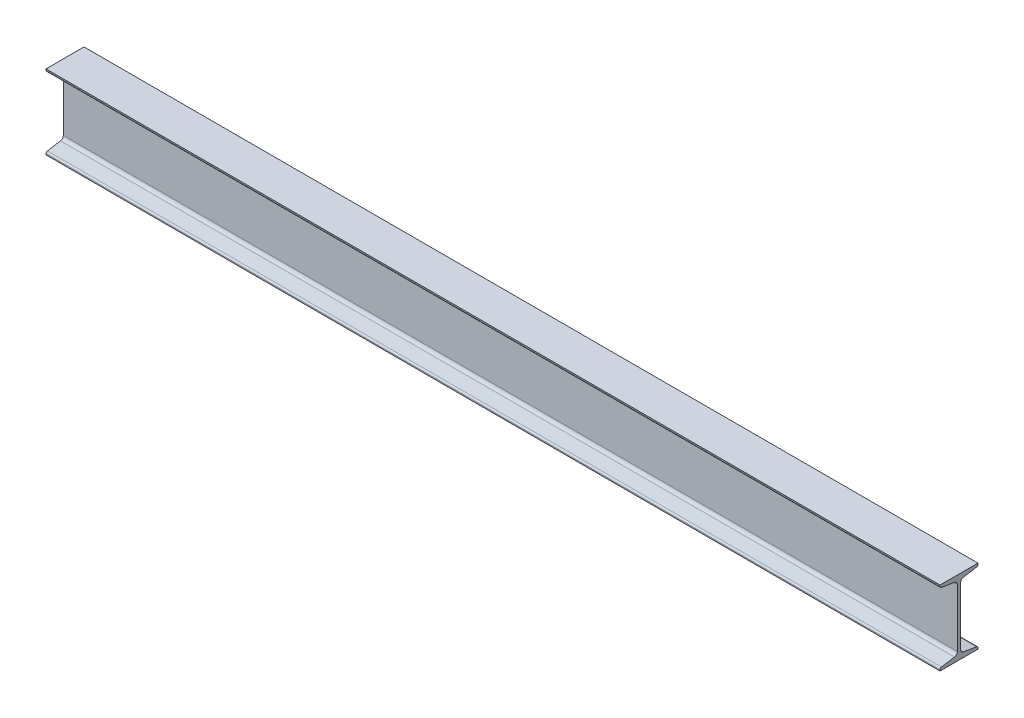
from build123d import *

# Parameters (mm, degrees)
BASE_DEPTH = 2400
FILLET1_R  = 9
FILLET2_R  = 4.5


with BuildPart() as part:
    # Sketch1 → Base (new body)
    with BuildSketch(Plane(origin=(0, 0, 0), x_dir=(0, 0, -1), z_dir=(1, 0, 0))):
        Polygon((-51, 0), (51, 0), (51, 6.775), (4.5, 14.525), (4.5, 185.475), (51, 193.225), (51, 200), (-51, 200), (-51, 193.225), (-4.5, 185.475), (-4.5, 14.525), (-51, 6.775), align=None)
    extrude(amount=BASE_DEPTH)

    # Fillet1
    fillet1_edges = [part.edges().sort_by_distance(p)[0] for p in [
        (1200, 14.525, 4.5),
        (1200, 185.475, 4.5),
        (1200, 185.475, -4.5),
        (1200, 14.525, -4.5),
    ]]
    fillet(fillet1_edges, radius=FILLET1_R)

    # Fillet2
    fillet2_edges = [part.edges().sort_by_distance(p)[0] for p in [
        (1200, 6.775, 51),
        (1200, 193.225, 51),
        (1200, 193.225, -51),
        (1200, 6.775, -51),
    ]]
    fillet(fillet2_edges, radius=FILLET2_R)


solid = part.part
